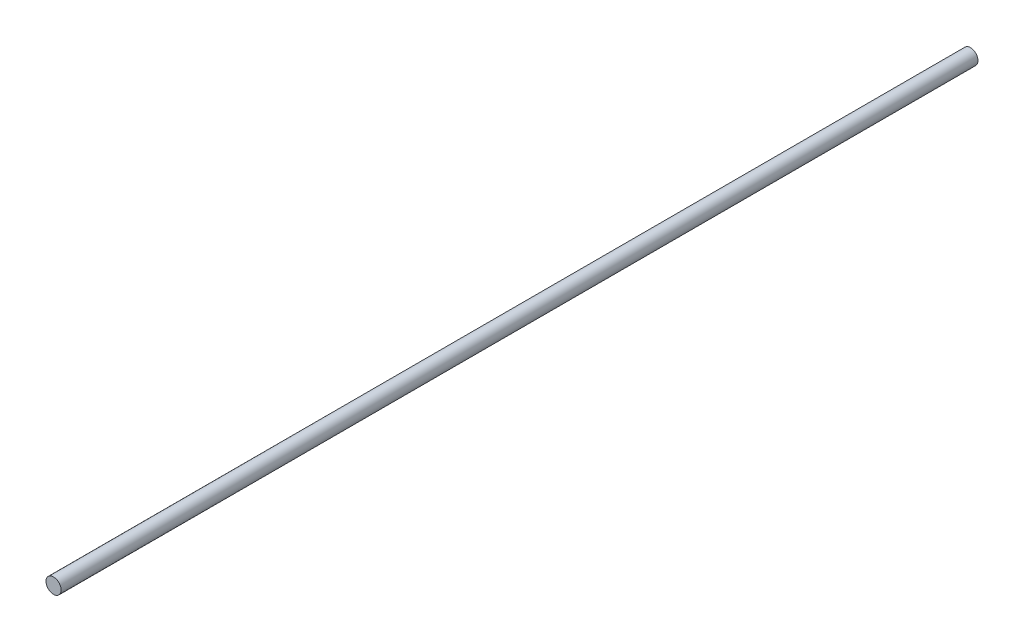
from build123d import *

# Parameters (mm, degrees)
SKETCH_1_R      = 8
EXTRUDE_1_DEPTH = 485


with BuildPart() as part:
    # 草图1 → 凸台-拉伸1 (new, symmetric)
    with BuildSketch(Plane.XY):
        Circle(SKETCH_1_R)
    extrude(amount=EXTRUDE_1_DEPTH, both=True)


solid = part.part
